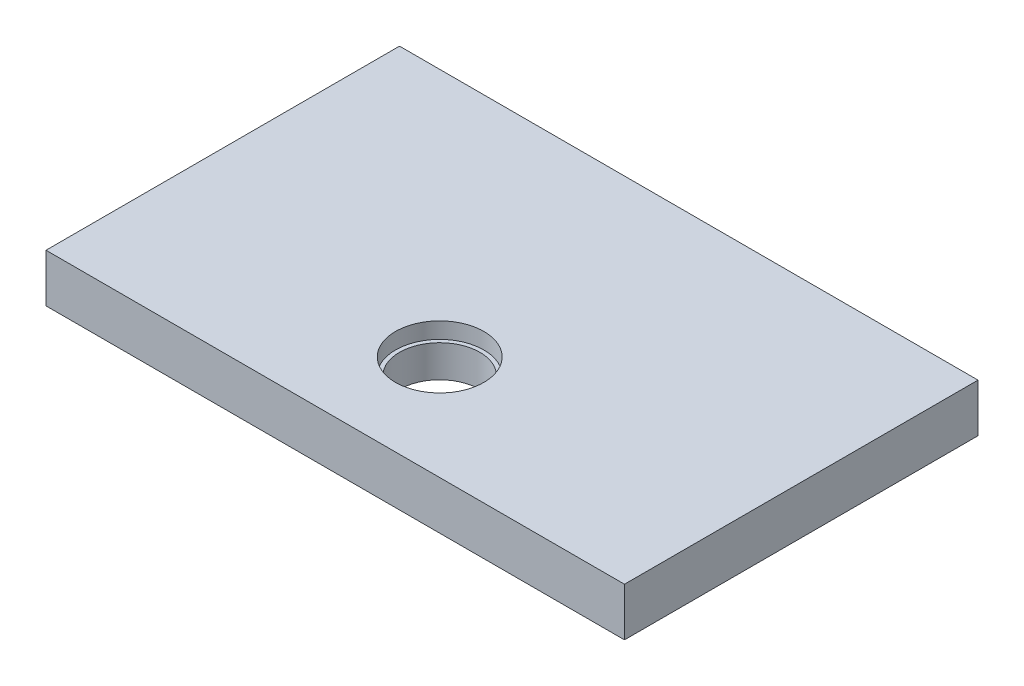
from build123d import *

# Parameters (mm, degrees)
SKETCH_1_W          = 360
SKETCH_1_H          = 220
EXTRUDE_1_DEPTH     = 30
SKETCH_2_R          = 27.5
CUT_EXTRUDE_1_DEPTH = 10
SKETCH_3_R          = 25
CUT_EXTRUDE_2_DEPTH = 214.072757527


with BuildPart() as part:
    # 草图1 → 凸台-拉伸1 (new body)
    with BuildSketch(Plane(origin=(0, 0, 0), x_dir=(1, 0, 0), z_dir=(0, 1, 0))):
        Rectangle(SKETCH_1_W, SKETCH_1_H)
    extrude(amount=EXTRUDE_1_DEPTH)

    # 草图2 → 切除-拉伸1 (cut)
    with BuildSketch(Plane(origin=(0, 30, 0), x_dir=(1, 0, 0), z_dir=(0, 1, 0))):
        with Locations(Location((0, -45, 0), (0, 0, 270))):
            Circle(SKETCH_2_R)
    extrude(amount=-CUT_EXTRUDE_1_DEPTH, mode=Mode.SUBTRACT)

    # 草图3 → 切除-拉伸2 (cut, through all)
    with BuildSketch(Plane(origin=(0, 30, 0), x_dir=(1, 0, 0), z_dir=(0, 1, 0))):
        with Locations(Location((0, -45, 0), (0, 0, 270))):
            Circle(SKETCH_3_R)
    extrude(amount=-CUT_EXTRUDE_2_DEPTH, mode=Mode.SUBTRACT)


solid = part.part
